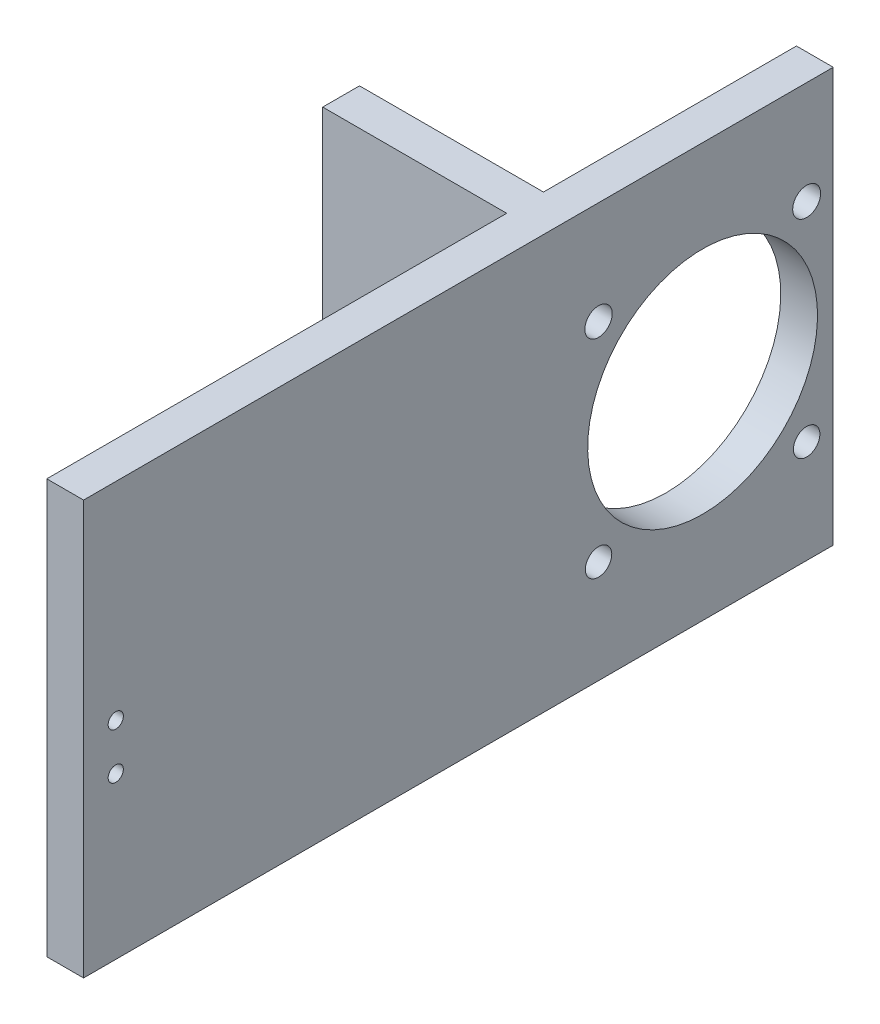
from build123d import *

# Parameters (mm, degrees)
SKETCH1_W             = 120
SKETCH1_H             = 90
SKETCH1_R             = 40
BOSS_EXTRUDE1_DEPTH   = 8
SKETCH3_W             = 8
SKETCH3_H             = 90
BOSS_EXTRUDE2_DEPTH   = 50
SKETCH4_W             = 8
SKETCH4_H             = 90
BOSS_EXTRUDE3_DEPTH   = 100
SKETCH5_W             = 178.684775764
SKETCH5_H             = 148.432517326
CUT_EXTRUDE1_DEPTH    = 156.32224567
SKETCH6_W             = 8
SKETCH6_H             = 90
BOSS_EXTRUDE4_DEPTH   = 55
SKETCH7_R             = 3.03642696
SKETCH7_R_2           = 2.873850802
SKETCH7_R_3           = 2.874430555
SKETCH7_R_4           = 2.981394427
SKETCH7_R_5           = 24.990861791
CUT_EXTRUDE2_DEPTH    = 35
M4_TAPPED_HOLE1_D     = 3.3
M4_TAPPED_HOLE1_DEPTH = 10.1
M4_TAPPED_HOLE1_TIP   = 0.991420021


with BuildPart() as part:
    # Sketch1 → Boss-Extrude1 (new body)
    with BuildSketch(Plane.XY):
        Rectangle(SKETCH1_W, SKETCH1_H)
        Circle(SKETCH1_R, mode=Mode.SUBTRACT)
    extrude(amount=BOSS_EXTRUDE1_DEPTH)

    # Sketch3 → Boss-Extrude2 (add)
    with BuildSketch(Plane.ZY.offset(60)):
        with Locations((4, 0)):
            Rectangle(SKETCH3_W, SKETCH3_H)
    extrude(amount=BOSS_EXTRUDE2_DEPTH)

    # Sketch4 → Boss-Extrude3 (add)
    with BuildSketch(Plane.XY.offset(8)):
        with Locations((-66, 0)):
            Rectangle(SKETCH4_W, SKETCH4_H)
    extrude(amount=BOSS_EXTRUDE3_DEPTH)

    # Sketch5 → Cut-Extrude1 (cut, through all)
    with BuildSketch(Plane.XY.offset(8)):
        with Locations((27.342387882, -29.216258663)):
            Rectangle(SKETCH5_W, SKETCH5_H)
    extrude(amount=-CUT_EXTRUDE1_DEPTH, mode=Mode.SUBTRACT)

    # Sketch6 → Boss-Extrude4 (add)
    with BuildSketch(Plane(origin=(0, 0, 0), x_dir=(-1, 0, 0), z_dir=(0, 0, -1))):
        with Locations((66, 0)):
            Rectangle(SKETCH6_W, SKETCH6_H)
    extrude(amount=BOSS_EXTRUDE4_DEPTH)

    # Sketch7 → Cut-Extrude2 (cut)
    with BuildSketch(Plane.ZY.offset(70)):
        with Locations(Location((-49.227416998, 22.627416998, 0), (0, 0, 270))):
            Circle(SKETCH7_R)
        with Locations(Location((-49.227416998, -22.627416998, 0), (0, 0, 270))):
            Circle(SKETCH7_R_2)
        with Locations(Location((-3.972583002, -22.627416998, 0), (0, 0, 270))):
            Circle(SKETCH7_R_3)
        with Locations(Location((-3.972583002, 22.627416998, 0), (0, 0, 270))):
            Circle(SKETCH7_R_4)
        with Locations(Location((-26.59999988, 0.009138209, 0), (0, 0, 270))):
            Circle(SKETCH7_R_5)
    extrude(amount=-CUT_EXTRUDE2_DEPTH, mode=Mode.SUBTRACT)

    # M4 Tapped Hole1
    with Locations(Plane.ZY.offset(70)):
        with Locations((101, 0), (101, -10)):
            Hole(M4_TAPPED_HOLE1_D / 2, depth=M4_TAPPED_HOLE1_DEPTH)
            with Locations((0, 0, -(M4_TAPPED_HOLE1_DEPTH + M4_TAPPED_HOLE1_TIP / 2))):  # 118° drill point
                Cone(0, M4_TAPPED_HOLE1_D / 2, M4_TAPPED_HOLE1_TIP, mode=Mode.SUBTRACT)


solid = part.part
